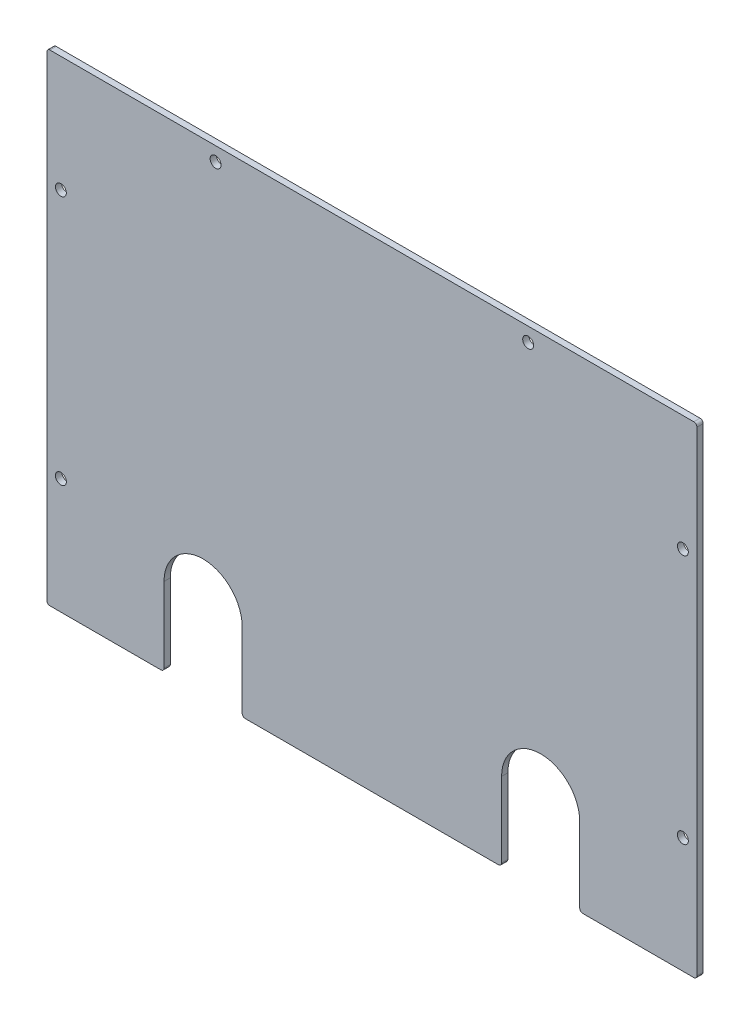
SolidWorks part; units mm, degrees
ref_plane "前视基准面" through (0, 0, 0) normal (0, 0, 1) x (1, 0, 0)
ref_plane "上视基准面" through (0, 0, 0) normal (0, 1, 0) x (1, 0, 0)
ref_plane "右视基准面" through (0, 0, 0) normal (1, 0, 0) x (0, 0, -1)
sketch "草图1" plane through (0, 0, 0) normal (0, 0, 1) x (1, 0, 0)
  line L1 (208, -154) -> (-208, -154)
  line L2 (208, -154) -> (208, 154)
  line L3 (208, 154) -> (-208, 154)
  line L4 (-208, -154) -> (-208, 154)
  line L5 (208, -154) -> (-208, 154) construction
  line L6 (208, 154) -> (-208, -154) construction
  point P0 (0, 0)
  dimension "D1" = 416
  dimension "D2" = 308
extrude "凸台-拉伸1" add sketch "草图1" along normal blind 4
fillet "圆角1" radius 2 4 edges at (208, 154, 2) (208, -154, 2) (-208, -154, 2) (-208, 154, 2)
sketch "草图2" plane through (0, 0, 4) normal (0, 0, 1) x (1, 0, 0)
  line L0 (-108, -154) -> (-108, -104) construction
  line L1 (-206, -154) -> (206, -154) construction
  line L2 (-133, -154) -> (-133, -104)
  line L3 (-83, -154) -> (-83, -104)
  line L4 (-208, 152) -> (-208, -152) construction
  arc A0 (-133, -154) -> (-83, -154) centre (-108, -154) ccw
  arc A1 (-83, -104) -> (-133, -104) centre (-108, -104) ccw
  point P4 (-108, -129)
  dimension "D1" = 50
  dimension "D2" = 100
  dimension "D3" = 50
extrude "切除-拉伸1" cut sketch "草图2" against normal up to next
mirror "镜向1" about plane through (0, 0, 0) normal (1, 0, 0) of "切除-拉伸1"
fillet "圆角2" radius 2 4 edges at (133, -154, 2) (83, -154, 2) (-83, -154, 2) (-133, -154, 2)
hole_wizard "M6 间隙孔1" positions "草图3" profile "草图4" hole size "M6" standard "GB" end condition up to next
sketch "草图3" plane through (0, 0, 4) normal (0, 0, 1) x (1, 0, 0)
  line L0 (-199, 80) -> (-199, -80) construction
  line L3 (-208, 0) -> (-199, 0) construction
  line L4 (-208, 152) -> (-208, -152) construction
  point P0 (-199, 80)
  point P2 (-199, -80)
  dimension "D1" = 160
  dimension "D2" = 9
sketch "草图4" plane through (-199, 80, 4) normal (1, 0, 0) x (0, -1, 0)
  line L0 (0, 0) -> (0, 4)
  line L1 (0, 4) -> (3.5, 4)
  line L2 (3.5, 4) -> (3.5, 0)
  line L5 (3.5, 0) -> (0, 0)
  line L11 (0, -6.35) -> (0, 107.95) construction
  dimension "通孔孔直径" = 7
  dimension "通孔孔深度" = 4
mirror "镜向2" about plane through (0, 0, 0) normal (1, 0, 0) of "M6 间隙孔1"
hole_wizard "M6 间隙孔2" positions "草图5" profile "草图6" hole size "M6" standard "GB" end condition up to next
sketch "草图5" plane through (0, 0, 4) normal (0, 0, 1) x (1, 0, 0)
  line L0 (-100, 145) -> (100, 145) construction
  line L3 (0, 145) -> (0, 154) construction
  line L4 (206, 154) -> (-206, 154) construction
  point P0 (-100, 145)
  point P2 (100, 145)
  dimension "D1" = 9
  dimension "D2" = 200
sketch "草图6" plane through (-100, 145, 4) normal (1, 0, 0) x (0, -1, 0)
  line L0 (0, 0) -> (0, 4)
  line L1 (0, 4) -> (3.5, 4)
  line L2 (3.5, 4) -> (3.5, 0)
  line L5 (3.5, 0) -> (0, 0)
  line L11 (0, -6.35) -> (0, 107.95) construction
  dimension "通孔孔直径" = 7
  dimension "通孔孔深度" = 4
